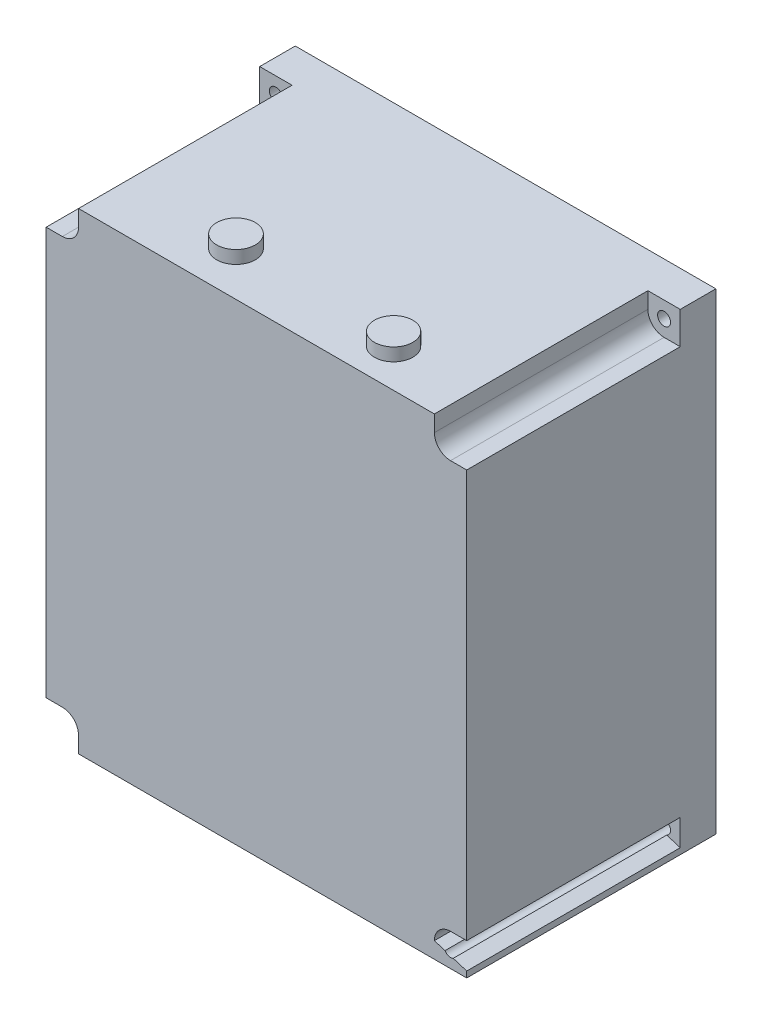
from build123d import *

# Parameters (mm, degrees)
SKETCH1_W           = 130
SKETCH1_H           = 146
SKETCH1_R           = 2
BOSS_EXTRUDE1_DEPTH = 77
CUT_EXTRUDE2_DEPTH  = 66
SKETCH4_R           = 5.985806468
SKETCH4_R_2         = 5.936967647
BOSS_EXTRUDE3_DEPTH = 150


with BuildPart() as part:
    # Sketch1 → Boss-Extrude1 (new body)
    with BuildSketch(Plane.XY):
        with Locations((65, 73)):
            Rectangle(SKETCH1_W, SKETCH1_H)
        with Locations((5, 141)):
            Circle(SKETCH1_R, mode=Mode.SUBTRACT)
        with Locations((125, 141)):
            Circle(SKETCH1_R, mode=Mode.SUBTRACT)
        with Locations((125, 5)):
            Circle(SKETCH1_R, mode=Mode.SUBTRACT)
        with Locations((5, 5)):
            Circle(SKETCH1_R, mode=Mode.SUBTRACT)
    extrude(amount=BOSS_EXTRUDE1_DEPTH)

    # Sketch3 → Cut-Extrude2 (cut)
    with BuildSketch(Plane.XY.offset(77)):
        with BuildLine():
            Line((120, 141), (120, 146))
            Line((120, 146), (146, 160))
            Line((146, 160), (130, 136))
            Line((130, 136), (125, 136))
            ThreePointArc((125, 136), (121.464466094, 137.464466094), (120, 141))
        make_face()
        with BuildLine():
            Line((10, 141), (10, 146))
            Line((10, 146), (0, 160))
            Line((0, 160), (0, 136))
            Line((0, 136), (5, 136))
            ThreePointArc((5, 136), (8.535533906, 137.464466094), (10, 141))
        make_face()
        with BuildLine():
            Line((10, 5), (10, 0))
            Line((10, 0), (0, 0))
            Line((0, 0), (0, 10))
            Line((0, 10), (5, 10))
            ThreePointArc((5, 10), (8.535533906, 8.535533906), (10, 5))
        make_face()
        with BuildLine():
            Line((120, 5), (136, 0))
            Line((136, 0), (146, 0))
            Line((146, 0), (130, 10))
            Line((130, 10), (125, 10))
            ThreePointArc((125, 10), (121.464466094, 8.535533906), (120, 5))
        make_face()
    extrude(amount=-CUT_EXTRUDE2_DEPTH, mode=Mode.SUBTRACT)

    # Sketch4 → Boss-Extrude3 (add)
    with BuildSketch(Plane(origin=(0, 0, 0), x_dir=(-1, 0, 0), z_dir=(0, -1, 0))):
        with Locations(Location((-45.096991408, -63.420422251, 0), (0, 0, 90))):
            Circle(SKETCH4_R)
        with Locations(Location((-95.564941336, -65.16467674, 0), (0, 0, 90))):
            Circle(SKETCH4_R_2)
    extrude(amount=-BOSS_EXTRUDE3_DEPTH)


solid = part.part
